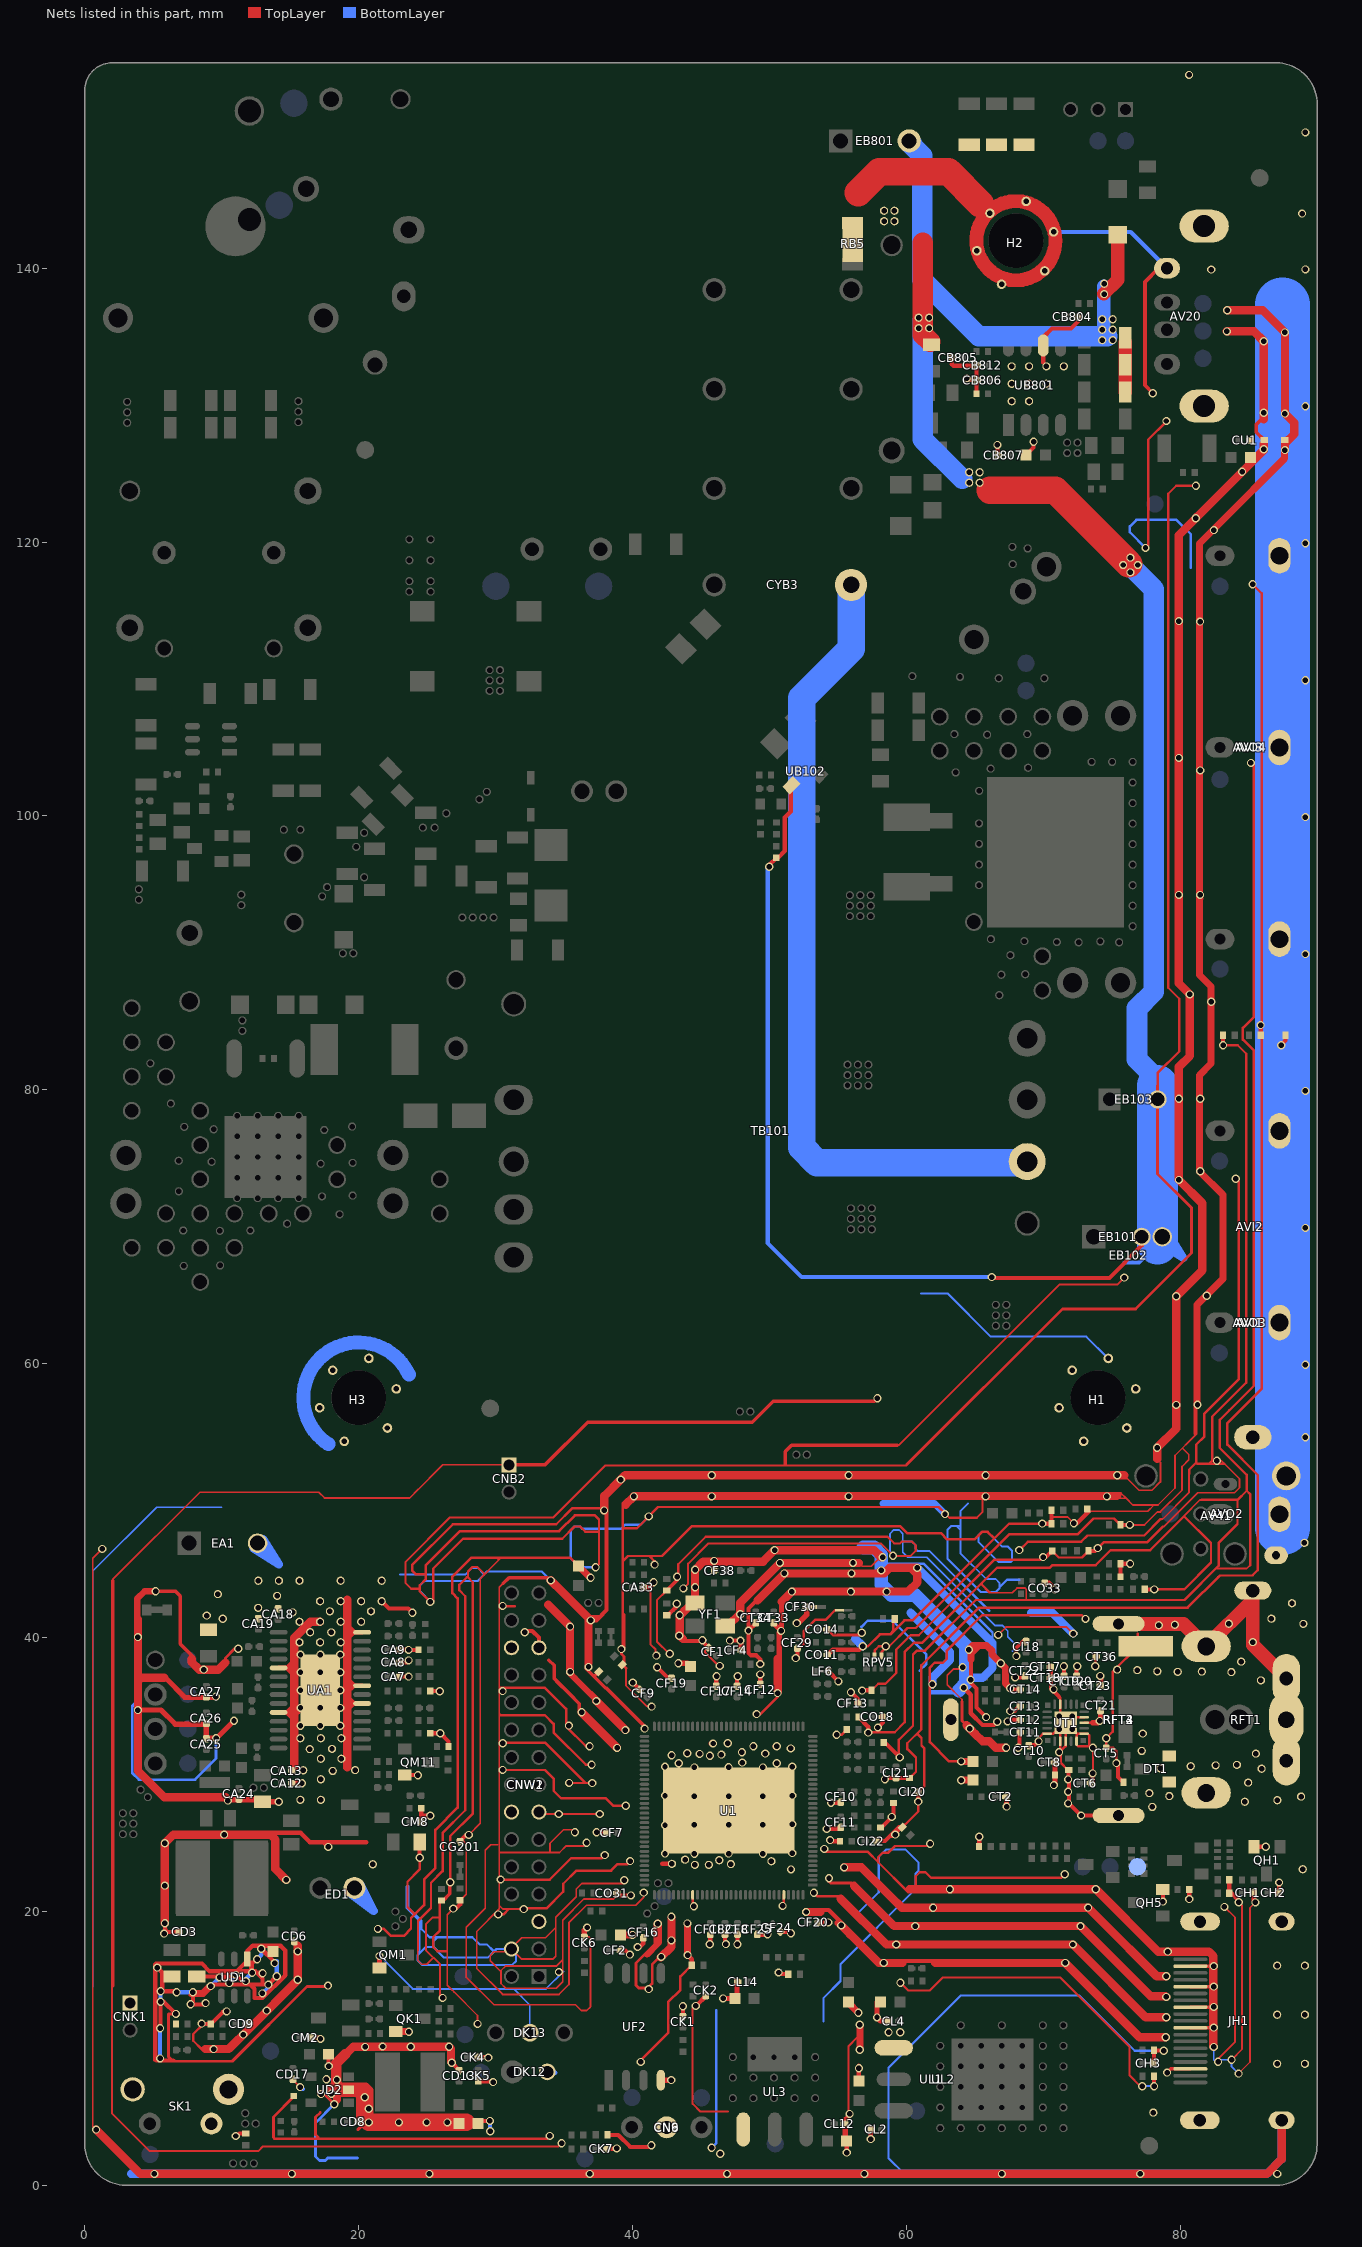
[diagram p0: the nets of this part, all layers, seen from the top]
# Altium PCB MISC116569.PcbDoc (part 8 of 15)
Units mm, origin at the board's own origin, x right, y up, seen from the top; angles counter-clockwise.
Board outline 90 x 155 mm, 2 copper layers (TopLayer, BottomLayer), stack 1.571 mm thick; 527 components, 277 nets, 2450 pads, 649 vias.

## Via types
v1: diameter 0.6, hole 0.4, TopLayer to BottomLayer, tented both sides, 649 vias

## Nets (pads, with @x,y where several pads share a name; then routed paths per layer and width w, separated by ;. In a path a pad name is that pad's centre, name@x,y a point inside that pad or via, vN(x,y) a via of type N, cw(c..) or ccw(c..) an arc to the next point about the centre after c; other vN are vias at no path point) (continued)
GND: AV20.4 AV20.5 AV20.6 AV41.1 AV41.2 AVI1.2 AVI1.4 AVI1.6 AVI2.2 AVI2.4 AVI3.2 AVI3.4 AVI3.6 AVO2.4 AVO2.5 AVO3.2 AVO3.4 AVO3.6 AVO4.2 AVO4.4 AVO4.6 CA1.1 CA2.1 CA7.1 CA8.1 CA9.1 CA12.1 CA13.1 CA18.1 CA19.1 CA24.1 CA25.2@8.877,32.47 CA25.2@8.877,32.645 CA26.1 CA27.2@8.878,35.614 CA27.2@8.878,35.789 CA33.1 CB801.2 CB804.1 CB805.2@63.32,133.477 CB805.2@63.495,133.477 CB806.2@65.29,131.826 CB806.2@65.115,131.826 CB807.1 CB811.1 CB812.2@65.29,132.918 CB812.2@65.115,132.918 CD1.2 CD2.2 CD3.1 CD6.1 CD7.1 CD8.1 CD9.1 CD10.1 CD13.1 CD14.1 CD15.1 CD16.1 CD17.1 CF1.1 CF2.1 CF3.1 CF4.1 CF5.1 CF7.1 CF8.1 CF9.1 CF10.1 CF11.2@55.207,26.08 CF11.2@55.207,26.255 CF12.1 CF13.1 CF14.1 CF15.1 CF16.1 CF17.1 CF18.2@45.683,18.283 CF18.2@45.683,18.458 CF19.2@42.85,36.893 CF19.2@42.85,37.069 CF20.1 CF21.2@46.749,18.283 CF21.2@46.749,18.458 CF24.2@50.702,18.615 CF24.2@50.825,18.491 CF25.2@49.112,18.283 CF25.2@49.112,18.458 CF29.2@52.04,39.18 CF29.2@52.04,39.355 CF30.2@52.544,42.23 CF30.2@52.719,42.23 CF38.1 CG201.2@27.414,24.969 CG201.2@27.414,25.144 CH1.2@85.37,21.365 CH1.2@85.195,21.365 CH2.2@87.05,21.364 CH2.2@87.225,21.364 CH3.1 CI18.1 CI20.2@60.696,28.727 CI20.2@60.871,28.727 CI21.2@59.245,29.712 CI21.2@59.245,29.887 CI22.2@57.637,25.133 CI22.2@57.812,25.133 CK1.1 CK2.2@45.347,13.801 CK2.2@45.347,13.976 CK4.2@28.591,9.362 CK4.2@28.766,9.362 CK5.2@28.735,7.566 CK5.2@28.735,7.741 CK6.1 CK7.2@37.981,2.657 CK7.2@38.156,2.657 CL1.1 CL2.1 CL3.1 CL4.1 CL11.1 CL12.1 CL13.1 CL14.1 CM2.1 CM7.2 CM8.1 CN6.2 CN9.2 CNB2.1 CNK1.1 CNW1.4 CNW1.5 CNW1.13 CNW1.14 CNW1.25 CNW1.26 CNW2.4 CNW2.5 CNW2.13 CNW2.14 CNW2.25 CNW2.26 CO11.1 CO14.1 CO18.1 CO31.1 CO33.1 CT1.1 CT2.1 CT5.2@74.595,31.787 CT5.2@74.595,31.962 CT6.2@73.49,29.365 CT6.2@73.315,29.365 CT8.2@70.691,30.875 CT8.2@70.866,30.875 CT9.1 CT10.1 CT11.1 CT12.1 CT13.2@68.258,34.978 CT13.2@68.433,34.978 CT14.1 CT17.2@70.383,37.848 CT17.2@70.558,37.848 CT18.1 CT19.1 CT20.1 CT21.1 CT22.2@68.664,37.14 CT22.2@68.664,37.315 CT23.2@74.031,36.487 CT23.2@74.206,36.487 CT33.1 CT34.2@49.002,41.031 CT34.2@49.002,41.206 CT36.2@73.823,38.608 CT36.2@73.998,38.608 CT52.1 CU1.2@84.948,127.419 CU1.2@85.123,127.419 CU2.2 CYB3.2 D101.A D102.A DA31.A DA32.A DA33.A DB804.K DH1.A DH2.A DH3.A DH81.A DI1.A DI2.A DI3.A DI10.A DI11.A DK1.A DK3.A DK12.K DK13.2 DT1.1 DT1.3 DU1.A DU2.A DU3.A DU4.A DV3.A DV4.A DV5.A DV7.A DV8.A DV9.A EA1.2 EB101.2 EB102.2 EB103.2 EB801.2 ED1.2 GDT1.2 GND.1 H1.1 H1.2 H1.3 H1.4 H1.5 H1.6 H2.1 H2.2 H2.3 H2.4 H2.5 H2.6 H3.1 H3.2 H3.3 H3.4 H3.5 H3.6 JH1.2 JH1.5 JH1.8 JH1.11 JH1.17 JH1.20 JH1.21 JH1.22 JH1.23 LF6.1 LT1.1 LT4.1 pad.VIA5@5.85,21.882 pad.VIA5@5.85,24.977 pad.VIA5@9.722,43.167 pad.VIA5@10.173,25.603 pad.VIA5@12.68,44.149 pad.VIA5@12.662,42.164 pad.VIA5@14.18,44.149 pad.VIA5@14.046,43.04 pad.VIA5@15.68,39.649 pad.VIA5@15.68,41.149 pad.VIA5@15.68,44.149 pad.VIA5@15.173,41.831 pad.VIA5@15.743,28.143 pad.VIA5@15.743,32.643 pad.VIA5@15.951,30.302 pad.VIA5@16.429,31.852 pad.VIA5@16.454,40.386 pad.VIA5@17.18,39.649 pad.VIA5@17.18,41.149 pad.VIA5@17.18,42.649 pad.VIA5@17.243,28.143 pad.VIA5@17.243,29.643 pad.VIA5@17.243,31.143 pad.VIA5@17.243,32.643 pad.VIA5@17.902,41.91 pad.VIA5@18.004,40.373 pad.VIA5@18.055,31.864 pad.VIA5@18.68,39.649 pad.VIA5@18.68,41.149 pad.VIA5@18.68,42.649 pad.VIA5@18.68,44.149 pad.VIA5@18.105,30.251 pad.VIA5@18.743,31.143 pad.VIA5@18.743,32.643 pad.VIA5@19.744,30.315 pad.VIA5@20.18,41.149 pad.VIA5@20.18,42.649 pad.VIA5@20.902,41.91 pad.VIA5@21.032,23.437 pad.VIA5@21.68,42.649 pad.VIA5@21.68,44.149 pad.VIA5@42.883,23.47 pad.VIA5@43.836,23.774 pad.VIA5@44.559,23.393 pad.VIA5@45.575,23.393 pad.VIA5@46.337,23.736 pad.VIA5@47.188,23.457 pad.VIA5@50.147,23.66 pad.VIA5@58.369,143.435 pad.VIA5@58.369,144.197 pad.VIA5@59.131,143.435 pad.VIA5@59.131,144.197 pad.VIA5@60.896,135.623 pad.VIA5@60.896,136.385 pad.VIA5@61.658,135.623 pad.VIA5@61.658,136.385 pad.VIA5@64.587,124.333 pad.VIA5@64.587,125.095 pad.VIA5@65.349,124.333 pad.VIA5@65.349,125.095 pad.VIA5@67.691,130.289 pad.VIA5@67.691,131.559 pad.VIA5@67.691,132.829 pad.VIA5@68.961,130.289 pad.VIA5@68.961,131.559 pad.VIA5@68.961,132.829 pad.VIA5@70.231,131.559 pad.VIA5@70.231,132.829 pad.VIA5@71.501,132.829 pad.VIA5@74.303,134.747 pad.VIA5@74.303,135.509 pad.VIA5@74.303,136.271 pad.VIA5@74.443,138.87 pad.VIA5@74.443,138.108 pad.VIA5@75.065,134.747 pad.VIA5@75.065,135.509 pad.VIA5@75.065,136.271 pad.VIA5@75.395,37.655 pad.VIA5@75.829,118.326 pad.VIA5@76.367,117.787 pad.VIA5@76.367,118.865 pad.VIA5@76.868,37.617 pad.VIA5@76.906,118.326 pad.VIA5@77.96,27.622 pad.VIA5@77.186,31.712 pad.VIA5@77.745,28.639 pad.VIA5@78.037,5.309 pad.VIA5@78.329,37.529 pad.VIA5@78.443,40.894 pad.VIA5@78.532,30.442 pad.VIA5@79.205,28.423 pad.VIA5@79.611,40.932 pad.VIA5@79.815,37.49 pad.VIA5@80.767,30.594 pad.VIA5@81.58,37.516 pad.VIA5@82.583,30.658 pad.VIA5@83.556,41.006 pad.VIA5@83.739,37.478 pad.VIA5@84.145,30.696 pad.VIA5@84.455,38.24 pad.VIA5@84.722,28.003 pad.VIA5@84.963,29.4 pad.VIA5@85.3,39.662 pad.VIA5@85.53,31.521 pad.VIA5@85.898,36.868 pad.VIA5@85.941,30.416 pad.VIA5@86.665,41.375 pad.VIA5@87.079,8.865 pad.VIA5@87.079,12.452 pad.VIA5@87.079,16.04 pad.VIA5@87.097,28.118 pad.VIA5@88.163,42.5 pad.VIA5@88.824,28.384 pad.VIA5@88.946,23.076 pad.VIA5@88.997,40.996 pad.VIA5@89.073,46.914 pad.VIA5@89.111,8.865 pad.VIA5@89.111,12.452 pad.VIA5@89.111,16.04 QH1.E QH5.E QK1.E QM1.E QM11.E RA1.2 RA4.JP_2K RA5.JP_2K RA9.1 RA11.1 RA31.1 RA32.1 RB5.2 RB5.3 RB134.1 RB803.1 RB818.1 RB819.1 RB820.1 RB837.1 RB838.1 RB839.2 RD5.1 RD6.1 RD8.2 RF12.2 RF13.2 RF16.2 RFT1.2 RFT1.3 RFT1.4 RFT2.2 RFT2.3 RFT2.4 RFT2.5 RFT3.2 RFT3.3@75.5,41 RFT3.4@75.5,27 RFT3.5@63.25,34 RFT3.6 RFT3.7 RFT4.2 RFT4.3 RFT4.4 RFT4.5 RH59.1 RH82.2 RI18.1 RM12.2 RM15.2 RO4.1 RO18.1 RO22.1 RPV5.4 RPV5.6 RV1.1 RV3.1 RV5.1 SK1.1 SK1.3 SK1.4 TB101.8 TP_12VA-.1 TP_12VB-.1 U1.105 U1.124 U1.EPAD UA1.6 UA1.8 UA1.14 UA1.19 UA1.24 UA1.EPAD UB102.A UB801.6 UD1.1 UD2.2 UF2.4 UL1.1 UL2.1 UL3.1 UT1.2 UT1.4 UT1.5 UT1.11 UT1.18 UT1.21 UT1.22 UT1.24 UT1.EPAD YF1.2 YF1.4 | length 3652.6
  TopLayer w0.127: v1(0.826,4.064) 0.584,4.305 0.584,45.783 v1(1.27,46.469) ; 2.045,43.485 2.045,44.243 8.412,50.61 14.516,50.61 15.267,50.61 14.884,50.61 ; 14.719,50.61 14.884,50.61 ; 24.15,50.61 26.15,52.61 CNB2.1@30.988,52.61 ; 24.333,17.165 24.322,17.153 24.322,16.414 24.594,16.142 24.979,16.142 25.385,16.547 ; 24.366,50.825 23.731,50.19 17.514,50.19 17.095,50.61 14.884,50.61 ; 26.817,14.262 26.969,14.111 ; v1(26.909,20.203) 26.467,19.76 26.467,14.613 26.969,14.111 ; RF13.2@27.414,20.812 27.851,21.248 27.851,24.938 27.645,25.144 CG201.2@27.414,25.144 ; v1(28.037,25.58) 28.878,26.422 28.878,44.301 30.234,45.656 ; 28.244,45.811 30.079,45.811 30.234,45.656 ; v1(28.684,11.775) 28.684,12.395 26.969,14.111 ; 29.965,17.041 30.31,17.041 ; 30.158,24.867 29.639,24.867 29.248,24.475 29.248,20.232 27.864,18.847 27.864,15.192 29.883,13.172 35.839,13.172 36.254,12.758 36.66,12.758 ; 30.275,20.421 30.526,20.17 31.72,20.17 ; 30.313,24.297 33.091,24.297 ; 30.389,45.811 30.234,45.656 ; 30.399,15.588 29.604,16.383 29.604,16.769 29.876,17.041 30.31,17.041 ; 30.57,43.963 30.275,43.668 30.275,20.181 28.626,18.532 28.626,15.823 30.514,13.934 34.628,13.934 35.356,14.662 35.356,19.161 36.641,20.445 40.235,20.445 40.825,21.035 v1(40.825,21.37) ; 30.714,14.417 30.399,14.732 ; 33.256,24.297 33.091,24.297 ; 34.391,18.821 33.649,18.079 31.923,18.079 31.164,17.32 CNW2.4@31.164,17.251 ; v1(35.796,25.774) 35.609,25.961 34.963,25.961 33.972,24.971 33.972,24.365 33.904,24.297 34.145,24.297 ; CK6.1@36.49,18.136 36.805,18.136 36.931,18.009 36.931,13.03 36.66,12.758 ; v1(36.642,25.017) 36.703,25.017 36.466,24.78 35.155,24.78 34.672,24.297 34.145,24.297 ; 36.906,13.004 36.66,12.758 ; CO31.1@38.907,21.338 38.907,21.185 38.624,20.903 36.451,20.903 34.899,19.35 34.899,16.474 ; v1@39.299,22.037 38.679,22.037 ; v1(39.403,22.278) 39.162,22.037 38.679,22.037 ; 39.42,37.857 39.517,37.759 39.517,36.909 ; 39.517,37.296 39.517,36.909 ; 40.97,35.042 40.853,35.158 ; v1(41.394,34.952) 41.363,34.982 41.029,34.982 40.853,35.158 ; v1(43.37,30.811) v1@43.37,30.882 ; 56.54,45.443 56.777,45.207 57.439,45.207 v1@58.095,45.862 ; 57.526,46.383 57.712,46.197 ; 64.067,35.331 64.067,35.471 62.982,36.555 62.982,37.249 63.426,37.694 63.983,37.694 v1(64.11,37.821) ; v1(65.784,50.305) 65.926,50.163 76.063,50.163 ; 66.11,43.273 67.743,43.273 68.078,43.608 68.664,43.608 68.761,43.511 68.761,42.769 68.732,42.74 ; v1@66.54,40.353 v1(66.705,40.188) 67.276,40.759 68.567,40.759 ; 68.339,40.759 68.567,40.759 ; 70.544,48.796 71.775,48.796 v1(72.233,48.339) 72.571,48.339 73.455,49.223 77.628,49.223 78.084,49.679 78.378,49.679 ; 71.082,51.613 76.121,51.613 76.44,51.294 ; v1@72.004,40.465 71.824,40.645 ; v1(72.182,40.287) 71.824,40.645 ; 74.257,50.546 75.679,50.546 76.063,50.163 ; 75.921,51.813 76.44,51.294 ; v1(76.322,48.224) 77.391,48.224 78.337,49.171 78.553,49.171 80.129,50.747 80.129,52.481 80.628,52.98 80.628,53.366 80.188,53.806 ; 78.313,53.038 78.554,52.796 78.554,51.363 77.937,50.746 76.988,50.746 76.44,51.294 ; 78.613,48.656 78.72,48.656 80.637,50.573 80.637,51.971 ; 78.808,48.097 81.289,50.578 83.964,50.578 84.329,50.942 84.329,51.597 83.015,52.911 ; 79.091,47.698 80.288,48.894 ; 80.288,48.856 80.288,48.894 ; 81.11,54.778 79.621,53.288 79.621,50.922 78.378,49.679 ; 81.581,50.044 81.438,50.044 80.288,48.894 ; 82.329,52.911 83.015,52.911 ; 82.554,44.982 82.61,45.038 84.856,45.038 85.108,45.289 ; v1(82.677,52.908) 82.679,52.911 83.015,52.911 ; v1@82.705,9.07 v1(82.766,9.01) 82.766,9.237 84.006,10.476 84.006,19.23 ; v1@82.748,9.185 v1@82.804,9.129 ; 82.754,44.428 82.856,44.53 85.275,44.53 85.3,44.555 ; v1(83.227,20.325) 84.006,19.547 84.006,19.23 ; v1(83.752,9.159) 84.514,9.921 84.514,20.426 v1(84.277,20.663) ; 84.006,19.548 84.006,19.23 ; 84.185,48.277 84.185,50.044 ; v1(84.26,8.156) 85.098,8.994 85.098,20.259 v1(85.491,20.653) ; 30.31,17.041 30.953,17.041 CNW2.4@31.164,17.251 ; 30.399,14.732 30.399,15.677 30.726,16.004 34.429,16.004 34.899,16.474 ; 30.399,14.732 30.74,14.392 34.439,14.392 34.899,14.852 34.899,16.474 ; CNW2.4@31.164,17.251 31.903,16.512 34.171,16.512 34.391,16.732 34.391,19.56 35.883,21.053 35.883,21.628 36.292,22.037 38.679,22.037 ; 33.091,24.297 34.145,24.297 ; 39.517,36.909 39.517,36.494 40.853,35.158 ; 68.567,40.759 71.71,40.759 71.824,40.645 ; 76.063,50.163 76.546,49.679 78.378,49.679
  TopLayer w0.152: 1.994,14.834 1.994,5.23 4.737,2.487 12.668,2.487 13.013,2.832 34.587,2.832 v1(34.818,3.063) ; CD17.1@15.197,7.693 15.723,7.167 v1(15.723,7.163) ; 24.465,43.561 23.838,43.561 23.411,43.988 23.411,45.506 26.675,48.77 34.227,48.77 38.022,52.565 59.69,52.565 ; 25.933,19.545 25.386,19.545 24.905,19.064 24.905,17.165 25.946,16.123 25.946,13.864 v1(26.132,13.678) ; 28.345,44.022 28.345,44.04 27.986,44.4 27.986,44.816 28.318,45.148 28.665,45.148 29.17,44.644 ; v1@41.3,43.993 41.3,39.511 41.681,39.13 41.681,38.748 v1(41.745,38.684) ; 41.783,42.197 41.783,41.862 ; v1(42.726,38.811) 42.683,38.811 41.783,39.711 41.783,41.862 ; 42.942,43.883 DI11.A@42.489,43.431 ; v1(43.251,44.44) 43.34,44.351 v1@43.34,44.281 ; v1(43.721,43.588) 44.064,43.931 44.064,45.392 45.55,46.878 58.136,46.878 59.05,45.964 v1(59.025,45.964) 60.31,45.964 60.684,46.337 60.684,46.733 60.404,47.013 59.68,47.013 59.545,46.878 59.109,46.878 58.627,47.361 45.35,47.361 43.34,45.351 v1@43.34,44.281 ; v1@44.597,13.122 44.394,12.918 44.394,5.936 44.945,5.385 46.972,5.385 ; CF1.1@45.545,39.265 45.301,39.021 45.301,38.905 46.279,37.926 v1(46.364,37.926) ; v1@47.837,31.78 v1(47.993,31.624) v1@48.044,31.573 ; v1(50.96,20.399) 51.028,20.399 v1@51.049,20.42 ; v1@51.533,23.064 v1(51.575,23.064) ; v1@55.85,5.095 55.771,5.174 55.771,10.16 56.409,10.798 56.599,10.798 ; 59.343,54.053 59.451,54.053 71.172,65.773 75.413,65.773 v1(75.921,66.281) ; v1(59.571,14.785) 60.14,14.216 61.712,14.216 62.674,15.179 71.22,15.179 76.297,10.102 76.297,8.02 77.082,7.235 v1(77.22,7.235) ; 60.303,52.892 59.975,52.565 ; 60.681,21.618 60.685,21.623 60.685,22.56 60.98,22.855 61.397,22.855 61.796,22.456 71.313,22.456 v1(71.564,22.708) ; v1(62.822,49.012) 62.873,49.012 63.139,48.745 64.498,48.745 ; 63.52,48.745 64.498,48.745 ; 65.552,50.002 65.552,49.708 ; v1(65.784,50.305) 65.552,50.074 65.552,49.708 ; 41.783,41.862 41.783,42.724 DI11.A@42.489,43.431 ; DI11.A@42.489,43.431 v1@43.34,44.281 ; 59.69,52.565 59.975,52.565 ; 59.69,52.565 59.975,52.565 ; 64.498,48.745 65.146,48.745 65.552,49.151 65.552,49.708
  TopLayer w0.178: 8.796,9.944 8.53,9.944 7.925,10.55 7.925,11.04 8.657,11.773 RD6.1@9.204,11.773 ; v1(21.407,18.72) 21.852,18.72 22.36,18.212 23.301,18.212 23.825,18.736 23.825,19.511 24.775,20.461 24.775,22.333 25.602,23.16 25.602,25.95 27.227,27.576 27.227,42.857 26.848,43.236 26.848,44.451 28.208,45.811 ; 24.116,19.802 24.089,19.802 23.566,20.325 23.566,22.165 24.455,23.054 v1(24.455,23.914) ; 24.333,17.165 24.333,19.301 25.283,20.251 25.283,22.086 26.136,22.939 26.136,25.729 27.786,27.38 27.786,43.016 27.356,43.447 27.356,43.853 27.902,44.4 27.986,44.4 ; 24.892,44.666 24.833,44.607 24.194,44.607 23.906,44.895 23.906,45.301 26.88,48.275 34.432,48.275 35.581,49.424 v1@37.778,49.424 ; v1@25.451,42.658 25.451,43.053 ; RO22.1@26.056,20.784 25.933,20.662 25.933,19.545 25.933,18.603 25.451,18.121 25.451,17.391 25.753,17.089 26.433,17.089 26.441,17.081 ; 26.694,21.293 26.694,25.498 28.345,27.149 28.345,44.022 ; 27.793,47.767 28.372,47.767 ; 28.025,47.208 28.448,47.208 ; 28.23,45.811 30.869,45.811 ; v1@30.202,19.774 30.569,19.774 30.965,20.17 v1(32.063,20.17) ; v1@30.326,30.203 30.445,30.322 31.25,30.322 ; v1@30.326,32.286 v1@30.362,32.322 ; 30.326,34.343 30.347,34.322 33.607,34.322 34.234,33.695 34.234,33.072 36.596,30.711 v1(37.016,30.711) v1@37.016,30.597 ; 30.326,36.337 v1@30.341,36.322 ; v1@30.33,22.322 31.415,22.322 ; v1(30.361,22.327) 30.365,22.322 31.415,22.322 ; 30.389,45.811 30.869,45.811 ; v1(30.512,36.09) 30.341,36.261 v1@30.341,36.322 ; v1(30.513,30.328) 30.508,30.322 31.25,30.322 ; v1(30.513,42.304) 30.445,42.304 30.419,42.278 31.39,42.278 ; v1(30.518,32.283) 30.401,32.283 v1@30.362,32.322 ; 31.162,20.17 v1(32.063,20.17) ; 31.598,44.376 33.35,44.376 ; CNW2.13@33.164,27.251 33.305,27.11 35.611,27.11 ; v1(34.607,27.11) 35.611,27.11 ; v1(35.36,33.564) 35.208,33.564 v1@35.149,33.505 ; v1(35.369,29.375) 35.367,29.373 36.557,29.373 ; CF15.1@36.063,45.21 35.461,45.811 30.869,45.811 ; v1(36.863,32.057) 36.596,32.057 v1@35.149,33.505 ; v1(37.054,29.373) 36.557,29.373 ; v1(37.308,45.126) 37.554,45.372 37.554,48.624 37.262,48.916 35.791,48.916 34.643,47.767 28.372,47.767 ; 37.554,47.676 37.505,47.724 36.558,47.724 36.177,48.105 35.771,48.105 34.874,47.208 28.448,47.208 ; v1(37.601,27.11) 35.611,27.11 ; v1(37.968,24.107) 37.752,23.891 35.524,23.891 33.955,22.322 31.415,22.322 ; v1@38.877,31.788 v1(38.877,31.937) ; 39.281,49.79 39.281,47.981 ; 39.332,41.303 39.281,41.354 39.281,45.557 ; v1(39.511,27.72) 38.583,27.72 38.055,28.247 34.795,28.247 34.234,28.807 34.234,29.695 33.607,30.322 31.25,30.322 ; v1(39.822,23.675) 39.602,23.455 38.916,23.455 38.438,22.977 35.902,22.977 34.943,22.017 34.943,21.442 33.722,20.221 32.113,20.221 v1(32.063,20.17) ; v1(40.61,9.007) 40.546,9.07 42.604,11.128 42.604,13.367 43.497,14.26 43.497,15.248 D102.A@44.33,16.081 ; v1(41.186,48.844) 41.542,49.2 ; v1(41.613,45.329) 41.613,45.57 41.232,45.951 ; CF29.2@52.04,39.18 52.172,39.18 52.497,39.505 52.497,40.441 53.368,41.311 54.12,41.311 RA4.JP_2K@54.806,41.997 ; v1@53.977,24.434 54.069,24.342 54.432,24.342 ; v1(54,24.562) 54.22,24.342 54.432,24.342 ; v1(56.815,39.36) 57.193,39.36 58.065,40.232 58.836,40.232 59.855,41.252 60.452,41.252 67.518,48.317 v1(69.931,48.317) ; v1(57.213,33.058) 57.239,33.084 59.151,33.084 59.874,33.806 59.874,38.935 60.539,39.601 61.136,39.601 66.642,45.106 70.492,45.106 70.67,45.284 73.83,45.284 74.928,46.383 77.814,46.383 80.288,48.856 82.249,46.894 82.249,45.468 80.294,43.513 v1(78.1,43.513) ; DV7.A@57.462,36.144 57.944,36.627 ; RPV5.4@57.686,38.649 57.686,39.063 57.983,39.36 v1(58.491,39.36) ; RPV5.6@58.186,38.649 58.186,38.953 58.491,39.258 v1(58.491,39.36) ; 58.204,36.627 57.944,36.627 ; 58.825,40.257 59.029,40.461 DV8.A@59.029,41.351 ; v1@59.106,25.527 60.871,27.292 v1(60.871,28.016) ; v1(59.525,31.239) 59.459,31.306 59.459,32.529 60.483,33.554 60.483,38.754 60.77,39.042 61.368,39.042 65.066,42.74 80.312,42.74 82.808,45.236 82.808,46.9 84.185,48.277 ; RV1.1@60.236,29.731 60.702,30.197 60.702,31.223 60.072,31.853 60.072,32.273 60.068,32.277 61.093,33.301 61.093,37.977 65.297,42.181 80.543,42.181 82.867,44.505 ; 60.777,32.985 61.104,32.658 61.104,32.108 61.312,31.9 61.312,29.168 CI20.2@60.871,28.727 ; v1(61.735,24.943) 61.747,24.93 61.747,24.773 59.181,24.773 58.697,24.289 58.276,24.289 57.95,23.963 57.95,23.584 ; v1(61.908,36.591) 61.713,36.397 61.713,35.667 ; 62.708,21.618 62.492,21.402 60.131,21.402 57.95,23.584 ; v1@62.873,49.012 62.355,49.53 41.872,49.53 41.542,49.2 ; 64.646,47.17 64.562,47.17 ; CT52.1@64.876,30.952 63.121,30.952 61.713,32.36 61.713,35.667 ; 65.421,43.885 65.498,43.885 66.085,43.299 ; 66.4,47.199 66.4,47.254 65.937,47.717 65.53,47.717 64.983,47.17 64.562,47.17 ; v1(68.238,46.384) 68.266,46.384 68.871,46.988 72.765,46.988 73.226,47.45 77.37,47.45 78.571,48.65 ; v1(69.655,32.426) 69.655,32.654 69.973,32.972 UT1.18@70.282,32.972 ; v1(69.98,45.876) 69.769,45.665 66.41,45.665 60.905,40.159 60.308,40.159 59.264,39.116 59.264,37.414 58.477,36.627 57.944,36.627 ; UT1.18@70.074,32.972 UT1.18@70.282,32.972 ; RO4.1@70.652,46.319 71.128,45.843 72.829,45.843 DA33.A@73.305,46.319 ; 70.892,35.925 71.232,35.585 UT1.11@71.232,35.122 UT1.EPAD@71.232,34.172 ; UT1.EPAD@70.912,33.162 70.722,32.972 UT1.18@70.282,32.972 ; v1(71.158,31.62) 71.285,31.493 71.285,30.828 71.789,30.324 LT4.1@71.852,30.324 ; UT1.EPAD@71.232,33.372 UT1.21@71.232,32.422 71.232,31.872 70.98,31.62 71.186,31.62 71.632,32.066 UT1.22@71.632,32.422 UT1.EPAD@71.632,33.772 ; UT1.EPAD@72.406,33.04 72.473,32.972 UT1.2@72.982,32.972 73.248,32.972 73.343,32.877 73.343,32.052 ; UT1.4@72.982,33.772 v1@74.031,33.772 ; UT1.5@72.982,34.172 72.032,34.172 UT1.EPAD@71.632,33.772 ; v1(73.084,41.354) 72.815,41.622 65.529,41.622 62.957,39.051 62.957,38.445 62.67,38.158 62.064,38.158 61.713,37.807 61.713,35.667 ; v1@73.521,32.052 v1(73.63,31.943) 73.63,30.101 v1(73.604,30.076) ; v1@73.562,32.061 72.546,32.061 72.432,32.176 UT1.24@72.432,32.422 72.432,32.972 UT1.EPAD@71.632,33.772 ; v1(73.8,37.906) 73.823,37.882 CT36.2@73.823,38.608 ; v1(73.983,46.526) 74.398,46.942 77.581,46.942 78.736,48.097 ; v1@75.458,30.711 75.319,30.851 75.319,31.727 75.084,31.962 CT5.2@74.595,31.962 v1(74.595,32.641) 75.077,33.124 75.077,37.516 76.913,39.351 76.913,40.274 ; DI3.A@75.642,48.224 75.177,48.69 73.676,48.69 72.534,47.547 67.538,47.547 60.684,40.693 60.087,40.693 58.754,39.36 v1(58.491,39.36) ; v1(77.465,119.57) 77.656,119.761 77.656,127.471 78.989,128.804 v1(78.989,128.841) ; 78.349,80.315 78.349,81.224 79.929,82.804 79.929,86.647 79.129,87.447 79.129,123.532 79.714,124.117 v1(81.15,124.117) ; 80.662,51.971 80.662,52.26 81.162,52.759 ; 81.581,50.044 84.185,50.044 84.862,50.721 ; 82.329,53.872 82.329,54.066 ; v1(83.129,83.251) 84.205,83.251 84.824,82.632 84.824,58.62 82.329,56.125 82.329,54.066 ; 83.203,52.687 82.105,52.687 ; v1(84.049,73.508) 84.061,73.508 84.265,73.303 84.265,72.288 84.265,58.852 81.77,56.357 81.77,54.684 81.162,54.075 81.162,52.759 ; 85.108,45.289 85.108,50.476 84.862,50.721 ; v1(85.161,103.876) 85.187,103.876 85.383,103.679 85.383,102.809 ; v1(85.288,116.916) 85.942,116.263 DV3.A@85.942,84.032 ; 85.3,44.555 85.667,44.922 85.667,51.862 83.447,54.082 83.447,55.662 85.942,58.157 85.942,83.924 DV3.A@85.878,83.987 ; 85.383,103.279 85.383,102.809 ; 25.451,43.053 25.451,42.812 v1(25.235,42.596) 24.465,43.366 24.465,43.815 24.892,44.242 24.892,45.261 27.398,47.767 28.372,47.767 ; 25.451,43.053 25.451,45.029 27.63,47.208 28.448,47.208 ; v1@30.341,36.322 33.607,36.322 35.149,34.781 v1@35.149,33.505 ; v1@30.362,32.322 33.607,32.322 36.557,29.373 ; 39.281,45.557 39.281,47.981 ; 39.281,45.557 39.675,45.951 41.232,45.951 ; 39.281,47.981 40.322,47.981 41.542,49.2 ; 41.232,45.951 42.154,45.951 44.313,48.11 59.57,48.11 60.053,47.627 62.517,47.627 62.974,47.17 64.562,47.17 ; 54.432,24.342 57.191,24.342 57.95,23.584 ; 81.162,52.759 81.234,52.687 82.105,52.687 ; 82.105,52.687 82.329,52.911 82.329,54.066 ; 84.862,50.721 84.862,51.877 82.888,53.851 82.888,55.894 83.594,56.599 85.383,58.389 85.383,82.863 84.577,83.669 84.577,84.518 85.383,85.324 85.383,102.809
  TopLayer w0.203: v1(6.651,12.51) 6.117,12.51 6.117,9.385 6.447,9.055 10.773,9.055 16.221,14.503 17.686,14.503 v1(17.762,14.58) ; 10.196,37.92 10.477,38.202 ; 10.274,38.173 10.274,38.508 10.946,39.179 v1(11.214,39.179) ; 13.847,3.391 14.054,3.391 ; RD8.2@15.241,6.458 13.775,4.991 13.775,3.48 13.864,3.391 14.054,3.391 ; 17.202,5.321 16.858,4.977 16.858,3.69 17.043,3.505 17.043,3.391 ; v1(17.254,6.655) 17.483,6.655 v1(18.22,5.918) ; v1(18.016,6.68) 18.423,7.087 18.423,7.684 v1(18.41,7.696) ; 19.934,4.051 20.467,4.585 v1(20.745,4.585) ; 27.452,3.391 27.249,3.391 ; v1(33.955,3.597) 33.749,3.391 27.249,3.391 ; v1@36.584,37.975 v1@36.584,37.757 ; 36.584,41.62 36.584,41.252 ; 36.584,41.651 36.584,41.252 ; v1@36.698,37.643 v1@36.698,37.848 ; 38.102,36.293 38.048,36.293 v1@36.584,37.757 ; v1@39.196,39.157 v1(39.187,39.157) 39.187,38.802 39.37,38.619 ; DU3.A@39.259,38.018 39.37,38.129 39.37,38.619 ; 39.517,37.759 39.37,37.907 39.37,38.619 ; v1(41.181,14.328) 41.181,14.48 41.435,14.734 ; 41.969,17.922 40.262,16.216 40.262,14.6 40.457,14.404 41.105,14.404 41.435,14.734 ; v1(42.1,16.673) 42.1,16.774 42.489,17.163 ; v1(42.845,17.882) 42.845,17.52 42.489,17.163 ; v1@44.4,20.485 U1.105@44.4,21.207 ; v1@49.245,34.411 v1(49.064,34.411) 49.345,34.411 50.595,35.661 v1(50.595,35.942) ; v1@51.049,20.42 U1.124@51.049,21.207 ; v1(53.251,21.362) 53.518,21.096 55.032,21.096 55.21,20.918 ; CO14.1@54.243,40.592 54.645,40.189 56.261,40.189 ; v1(54.351,22.418) 54.351,22.164 54.454,22.061 55.97,22.061 56.174,21.858 ; v1(54.902,32.893) 55.252,32.893 RF12.2@55.646,33.287 ; v1(56.749,40.341) 56.597,40.189 56.261,40.189 ; v1@56.866,40.35 56.705,40.189 56.261,40.189 ; 60.023,52.613 71.405,63.995 76.746,63.995 80.823,68.072 80.823,71.387 78.349,73.861 78.349,80.315 ; 64.067,35.331 64.067,33.92 64.395,33.592 ; 14.054,3.391 17.043,3.391 ; 17.043,3.391 27.249,3.391 ; v1@36.584,37.757 36.584,41.252 ; 41.435,14.734 41.435,16.11 42.489,17.163
  TopLayer w0.254: 2.045,14.584 2.045,41.618 ; 2.045,43.887 2.045,41.618 ; 2.045,44.153 2.045,41.618 ; v1(5.169,43.383) 6.627,43.383 6.982,43.028 6.982,39.525 7.931,38.577 ; 7.931,38.386 7.931,38.577 ; 8.236,37.776 7.931,38.081 7.931,38.577 ; RO22.1@26.056,20.784 26.164,20.784 26.656,21.276 26.656,22.085 v1(26.694,22.123) ; 30.57,43.963 30.983,44.376 33.35,44.376 33.823,44.376 v1@34.168,44.031 ; CNB2.1@30.988,52.61 33.612,52.61 36.717,55.715 48.751,55.715 50.289,57.253 57.672,57.253 v1(57.887,57.468) ; 33.891,38.343 34.272,37.962 34.272,37.004 35.368,35.909 ; 34.45,36.826 35.368,35.909 ; v1@36.101,34.597 36.101,35.175 35.368,35.909 ; 37.197,37.179 37.206,37.179 DU4.A@37.541,37.514 ; DI11.A@42.489,43.431 43.251,44.193 v1(43.251,44.44) ; 51.143,52.642 51.143,53.581 51.615,54.053 59.343,54.053 ; v1(68.043,38.645) 68.008,38.679 68.008,39.216 68.549,39.757 CI18.1@68.745,39.757 ; v1(79.039,8.223) 79.316,8.5 JH1.17@80.742,8.5 ; JH1.11@80.742,11.5 82.448,11.5 v1(82.456,11.509) ; JH1.8@80.742,13 82.436,13 v1(82.456,13.02) ; JH1.5@80.742,14.5 82.45,14.5 v1(82.456,14.506) ; JH1.2@80.742,16 82.452,16 v1(82.456,16.004) ; 85.847,128.881 85.555,128.589 85.555,128.014 86.117,127.451 DU2.A@86.126,127.451
  TopLayer w0.279: v1@36.622,37.773 36.698,37.848 v1(36.787,37.848) ; 36.787,40.655 36.787,40.674 ; v1@36.787,41.412 36.881,41.506 37.619,41.506 38.113,42 ; v1(36.949,41.25) 37.362,41.25 38.113,42 ; 38.102,36.293 40.881,33.514 v1(40.881,33.347) ; 38.113,50.508 38.113,42 ; v1(39.187,39.157) 39.332,39.301 39.332,41.303 39.332,41.646 ; v1(78,130.874) 77.417,131.457 77.417,138.998 78.419,140 AV20.4@79.04,140